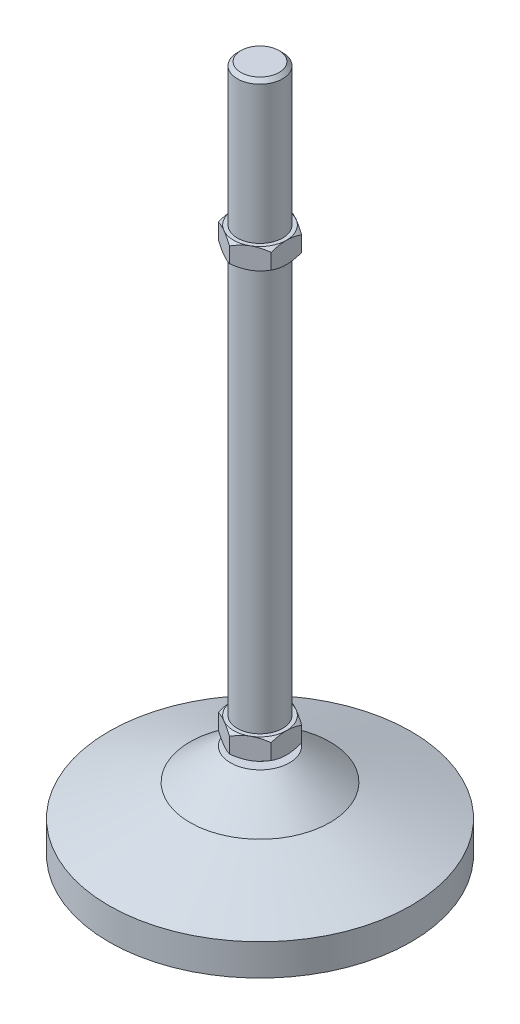
SolidWorks part; units mm, degrees
ref_plane "Front Plane" through (0, 0, 0) normal (0, 0, 1) x (1, 0, 0)
ref_plane "Top Plane" through (0, 0, 0) normal (0, 1, 0) x (1, 0, 0)
ref_plane "Right Plane" through (0, 0, 0) normal (1, 0, 0) x (0, 0, -1)
sketch "Sketch1" plane through (0, 0, 0) normal (1, 0, 0) x (0, 0, -1)
  line L0 (0, 0) -> (0, 182) construction
  line L1 (0, 182) -> (6, 182)
  line L2 (6, 182) -> (6, 144.5)
  line L3 (6, 144.5) -> (7, 144.5)
  line L4 (7, 144.5) -> (7, 138.9)
  line L5 (7, 138.9) -> (6, 138.9)
  line L6 (6, 138.9) -> (6, 25)
  line L8 (7, 32) -> (7, 26.4)
  line L12 (7.8, 25) -> (18.5333, 16.6667)
  line L13 (18.5333, 16.6667) -> (40, 8.3333)
  line L14 (40, 8.3333) -> (40, 0)
  line L15 (40, 0) -> (0, 0)
  line L16 (0, 4.1667) -> (6, 4.1667)
  line L17 (6, 4.1667) -> (6, 0)
  line L18 (36, 0) -> (36, 5.5953)
  line L19 (36, 5.5953) -> (20, 11.8065)
  line L21 (7.8, 25) -> (0, 25)
  line L22 (40, 8.3333) -> (40, 16.6667) construction
  line L23 (40, 16.6667) -> (40, 25) construction
  line L24 (20, 11.8065) -> (20, 0)
  line L25 (7.8, 25) -> (18.5333, 25) construction
  line L26 (18.5333, 25) -> (29.2667, 25) construction
  line L27 (29.2667, 25) -> (40, 25) construction
  line L28 (7, 26.4) -> (4.8, 26.4)
  line L29 (4.8, 26.4) -> (4.8, 25)
  circle A1 centre (0, 18.75) radius 9.7168
  point P19 (40, 4.1667)
  point P28 (20, 0)
  point P31 (7.44, 25)
  dimension "D1" = 8.3333
  dimension "A" = 150
  dimension "H" = 25
  dimension "M" = 12
  dimension "H1" = 32
  dimension "s" = 14
  dimension "D2" = 0.36
  dimension "D" = 80
  dimension "D3" = 6.25
  dimension "D4" = 5.6
  dimension "D5" = 37.5
  dimension "D6" = 4
  dimension "D7" = 4
  dimension "D8" = 14
  dimension "D9" = 1.8
  dimension "D10" = 5.6
  dimension "D11" = 9.6
sketch "Sketch2" plane through (0, 0, 0) normal (1, 0, 0) x (0, 0, -1)
  line L0 (0, 182) -> (6, 182) construction
  line L1 (4.8, 26.4) -> (4.8, 25) construction
  line L2 (4.8, 32) -> (4.8, 25)
  line L5 (7.8, 25) -> (0, 25) construction
  line L6 (7.8, 25) -> (4.8, 25)
  line L7 (6, 32) -> (4.8, 32)
  line L11 (7.8, 25) -> (18.5333, 16.6667) construction
  line L12 (18.5333, 16.6667) -> (40, 8.3333) construction
  line L13 (40, 8.3333) -> (40, 0) construction
  line L14 (40, 0) -> (0, 0) construction
  line L20 (0, 182) -> (6, 182)
  line L21 (6, 138.9) -> (6, 25) construction
  line L22 (6, 182) -> (6, 32)
  line L31 (7.8, 25) -> (18.5333, 16.6667)
  line L32 (18.5333, 16.6667) -> (40, 8.3333)
  line L33 (40, 8.3333) -> (40, 0)
  line L34 (40, 0) -> (0, 0)
  line L40 (0, 182) -> (0, 0)
revolve "Revolve1" add sketch "Sketch2" angle 360 mid plane about L40
cosmetic thread "Cosmetic Thread4" parameters "D2"=11.9
cosmetic thread "Cosmetic Thread5" parameters "D2"=9.5
chamfer "Chamfer1" distance 0.96 angle 45 1 edges at (0, 182, 6)
sketch "Sketch3" plane through (0, 0, 0) normal (0, 1, 0) x (1, 0, 0)
  line L1 (7, -4.0415) -> (7, 4.0415)
  line L2 (7, 4.0415) -> (0, 8.0829)
  line L3 (0, 8.0829) -> (-7, 4.0415)
  line L4 (-7, 4.0415) -> (-7, -4.0415)
  line L5 (-7, -4.0415) -> (0, -8.0829)
  line L6 (0, -8.0829) -> (7, -4.0415)
  circle A0 centre (0, 0) radius 7 construction
extrude "Boss-Extrude1" add sketch "Sketch3" along normal up to vertex (32 mm away) from vertex at 26.4 separate body starting at point (0, 26.4, -7)
sketch "Sketch8" plane through (0, 0, 0) normal (0, 1, 0) x (1, 0, 0)
  line L1 (7, -4.0415) -> (7, 4.0415)
  line L2 (7, 4.0415) -> (0, 8.0829)
  line L3 (0, 8.0829) -> (-7, 4.0415)
  line L4 (-7, 4.0415) -> (-7, -4.0415)
  line L5 (-7, -4.0415) -> (0, -8.0829)
  line L6 (0, -8.0829) -> (7, -4.0415)
  circle A0 centre (0, 0) radius 7 construction
extrude "Boss-Extrude2" add sketch "Sketch8" along normal up to vertex (144.5 mm away) from vertex at 138.9 separate body starting at point (0, 138.9, -7)
sketch "Sketch6" plane through (0, 32, 0) normal (0, 1, 0) x (1, 0, 0)
  line L0 (6.0622, 3.5) -> (7.9378, 4.5829) construction
  circle A0 centre (0, 0) radius 7
  circle A2 centre (0, 0) radius 9.1658
  point P6 (7, 4.0415)
extrude "Cut-Extrude4" cut sketch "Sketch6" against normal up to vertex (5.6 mm away) draft 55
sketch "Sketch7" plane through (0, 26.4, 0) normal (0, -1, 0) x (1, 0, 0)
  circle A0 centre (0, 0) radius 7 construction
  circle A2 centre (0, 0) radius 9.1658 construction
  circle A4 centre (0, 0) radius 9.1658
  circle A5 centre (0, 0) radius 7
extrude "Cut-Extrude5" cut sketch "Sketch7" against normal blind 5.6 draft 55
sketch "Sketch9" plane through (0, 144.5, 0) normal (0, 1, 0) x (1, 0, 0)
  line L0 (0, 7) -> (0, 9.1658) construction
  circle A0 centre (0, 0) radius 9.1658
  circle A1 centre (0, 0) radius 7
  point P8 (0, 8.0829)
extrude "Cut-Extrude6" cut sketch "Sketch9" against normal up to vertex (5.6 mm away) draft 55
sketch "Sketch10" plane through (0, 138.9, 0) normal (0, -1, 0) x (1, 0, 0)
  circle A0 centre (0, 0) radius 9.1658 construction
  circle A1 centre (0, 0) radius 9.1658
  circle A2 centre (0, 0) radius 7 construction
  circle A3 centre (0, 0) radius 7
extrude "Cut-Extrude7" cut sketch "Sketch10" against normal blind 5.6 draft 55
